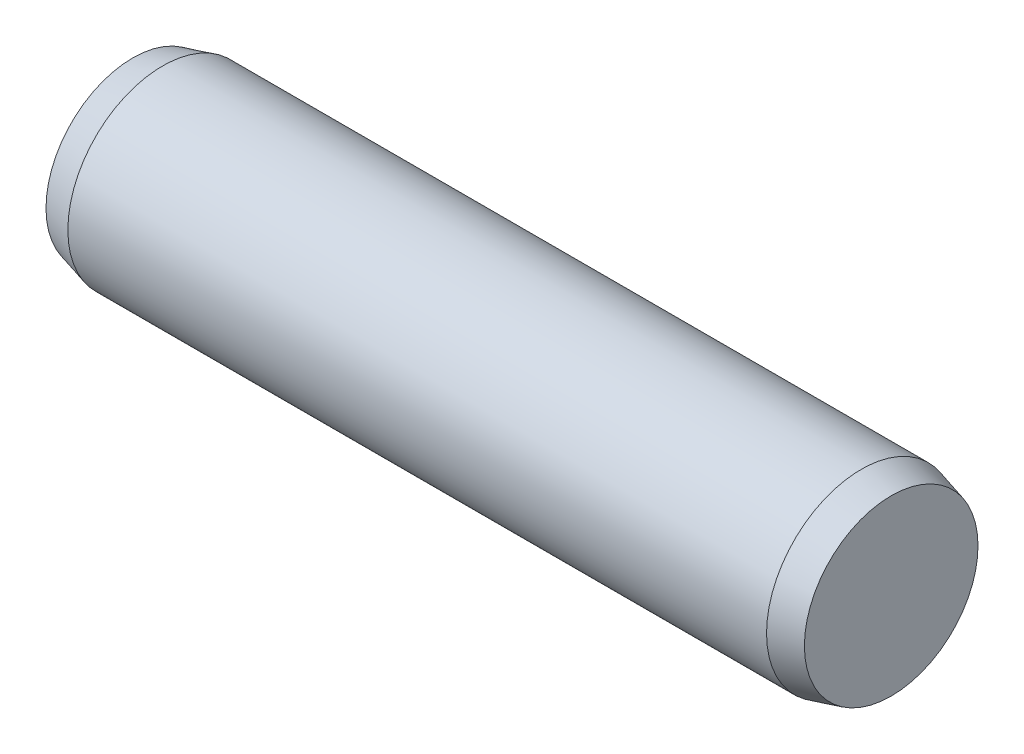
SolidWorks part; units mm, degrees
material "35钢"
ref_plane "Front" through (0, 0, 0) normal (0, 0, 1) x (1, 0, 0)
ref_plane "Top" through (0, 0, 0) normal (0, 1, 0) x (1, 0, 0)
ref_plane "Right" through (0, 0, 0) normal (1, 0, 0) x (0, 0, -1)
sketch "Sketch1" plane through (0, 0, 0) normal (0, 0, 1) x (1, 0, 0)
  line L0 (0, 0) -> (0.482, 0) construction
  line L1 (-1.63, 0) -> (14.37, 0)
  line L2 (-1, 2) -> (13.74, 2)
  line L3 (14.37, 1.8312) -> (14.37, 0)
  line L4 (13.74, 2) -> (14.37, 1.8312)
  line L5 (-1, -2) -> (13.74, -2) construction
  line L6 (-1, 2) -> (-1.63, 1.8312)
  line L7 (-1.63, 1.8312) -> (-1.63, 0)
  point P13 (6.37, 2)
revolve "Base-Revolve" add sketch "Sketch1" angle 360 about L0
equation "\"D2@Sketch1\" = \"c@Sketch1\""
